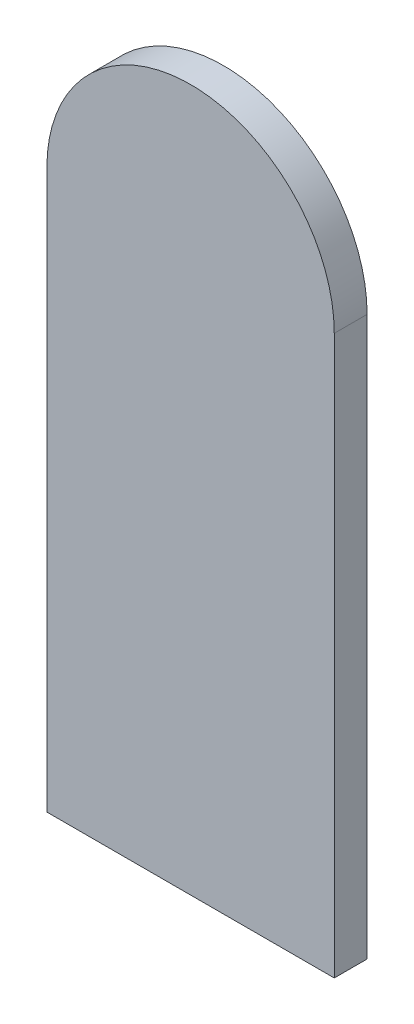
SolidWorks part; units mm, degrees
ref_plane "前视基准面" through (0, 0, 0) normal (0, 0, 1) x (1, 0, 0)
ref_plane "上视基准面" through (0, 0, 0) normal (0, 1, 0) x (1, 0, 0)
ref_plane "右视基准面" through (0, 0, 0) normal (1, 0, 0) x (0, 0, -1)
sketch "草图1" plane through (0, 0, 0) normal (0, 0, 1) x (1, 0, 0)
  line L0 (0, 0) -> (-17.5, 0)
  line L1 (-17.5, 0) -> (-17.5, 68)
  line L2 (17.5, 68) -> (17.5, 0)
  line L3 (17.5, 0) -> (0, 0)
  arc A0 (-17.5, 68) -> (17.5, 68) centre (0, 68) cw
  dimension "D1" = 35
  dimension "D2" = 68
extrude "凸台-拉伸1" add sketch "草图1" along normal blind 4
